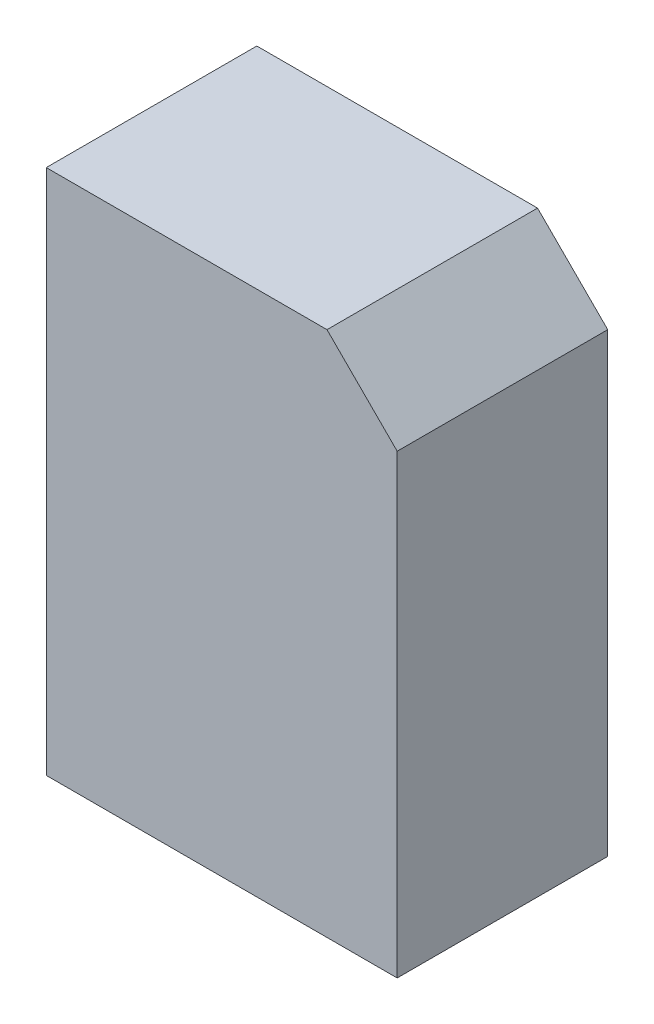
SolidWorks part; units mm, degrees
material "Q235A"
ref_plane "Front Plane" through (0, 0, 0) normal (0, 0, 1) x (1, 0, 0)
ref_plane "Top Plane" through (0, 0, 0) normal (0, 1, 0) x (1, 0, 0)
ref_plane "Right Plane" through (0, 0, 0) normal (1, 0, 0) x (0, 0, -1)
sketch "Sketch1" plane through (0, 0, 0) normal (0, 0, 1) x (1, 0, 0)
  line L1 (-500, 750) -> (500, 750)
  line L2 (-500, 750) -> (-500, -750)
  line L3 (-500, -750) -> (500, -750)
  line L4 (500, 750) -> (500, -750)
  line L5 (-500, 750) -> (500, -750) construction
  line L6 (-500, -750) -> (500, 750) construction
  point P0 (0, 0)
  dimension "D1" = 1000
  dimension "D2" = 1500
extrude "Boss-Extrude1" add sketch "Sketch1" along normal blind 600
chamfer "Chamfer1" distance 200 angle 45 1 edges at (500, 750, 300)
